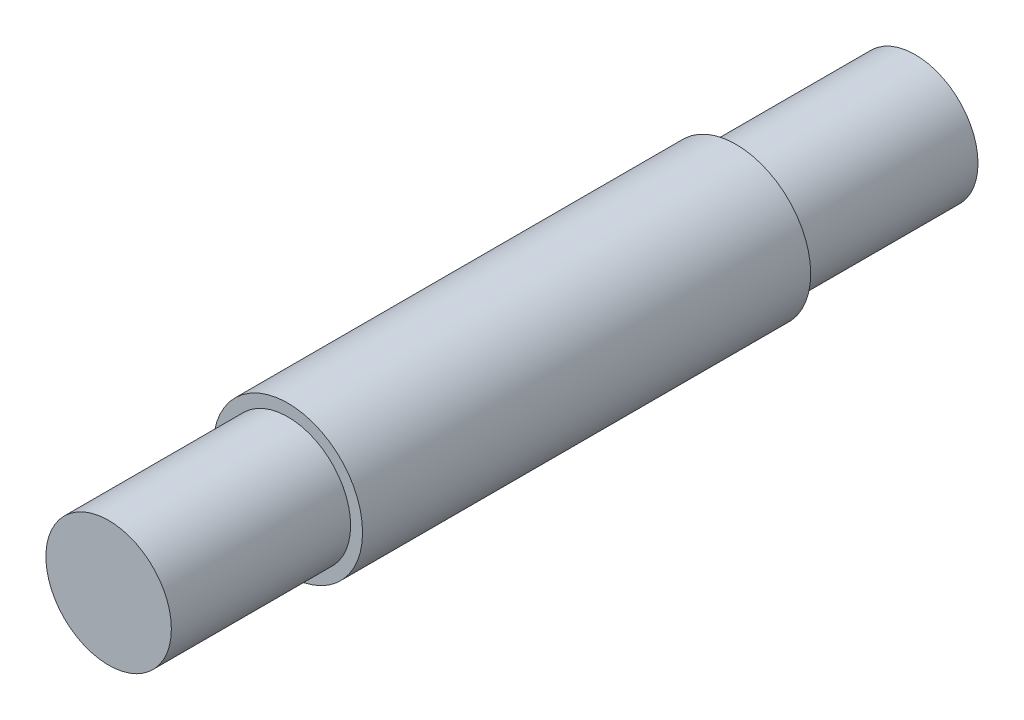
from build123d import *

# Parameters (mm, degrees)
SKETCH_1_R           = 25
BOSS_EXTRUDE_1_DEPTH = 75
SKETCH_2_R           = 21
BOSS_EXTRUDE_2_DEPTH = 60


with BuildPart() as part:
    # Sketch 1 → Boss-Extrude 1 (new, symmetric)
    with BuildSketch(Plane.XY):
        Circle(SKETCH_1_R)
    extrude(amount=BOSS_EXTRUDE_1_DEPTH, both=True)

    # Sketch 2 → Boss-Extrude 2 (add)
    with BuildSketch(Plane.XY.offset(75)):
        Circle(SKETCH_2_R)
    boss_extrude_2 = extrude(amount=BOSS_EXTRUDE_2_DEPTH)

    # Mirror 1: Boss-Extrude 2 across plane
    add(boss_extrude_2.mirror(Plane.XY))


solid = part.part
